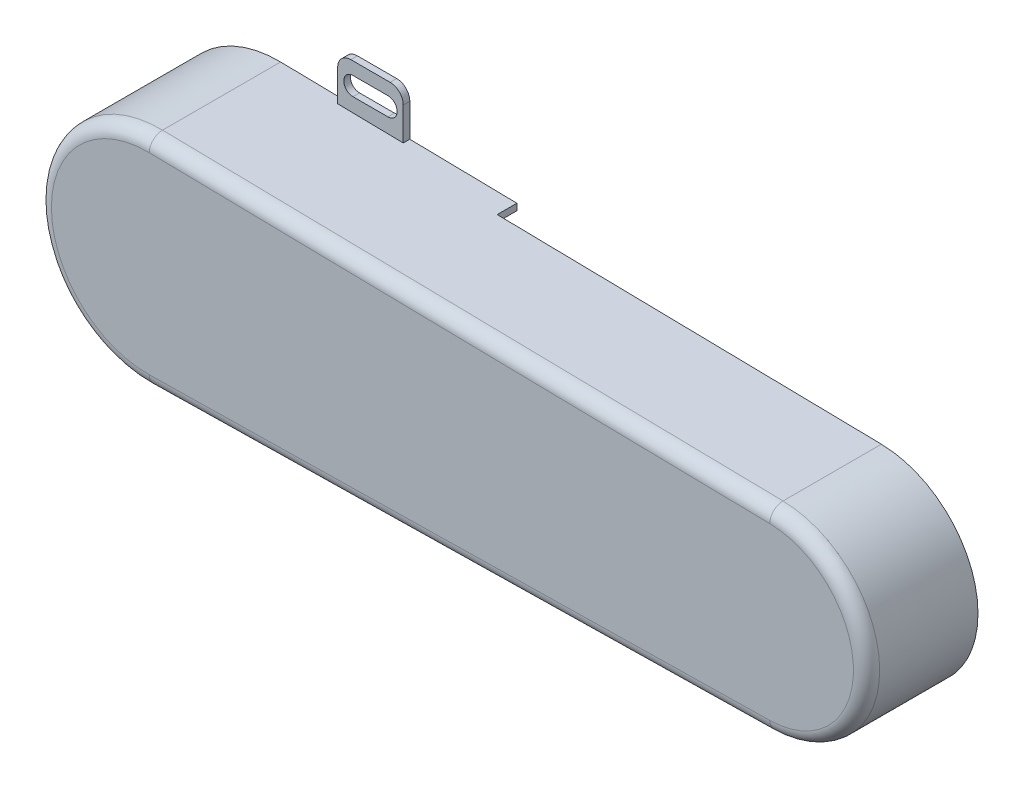
from build123d import *

# Parameters (mm, degrees)
EXTRUDE_1_DEPTH     = 30
SHELL_1_T           = -1.5
EXTRUDE_2_DEPTH     = 1.5
CUT_EXTRUDE_1_DEPTH = 1.5
FILLET_1_R          = 3
SKETCH_4_W          = 110
SKETCH_4_H          = 4.5
CUT_EXTRUDE_2_DEPTH = 30


with BuildPart() as part:
    # 草图1 → 凸台-拉伸1 (new body)
    with BuildSketch(Plane.XY):
        with BuildLine():
            Line((0.440140845, 24.99612522), (142.396126761, 22.496512698))
            ThreePointArc((142.396126761, 22.496512698), (164.5, 0), (142.396126761, -22.496512698))
            Line((142.396126761, -22.496512698), (0.440140845, -24.99612522))
            ThreePointArc((0.440140845, -24.99612522), (-25, 0), (0.440140845, 24.99612522))
        make_face()
    extrude(amount=EXTRUDE_1_DEPTH)

    # 抽壳1
    shell_1_openings = [part.faces().sort_by_distance(p)[0] for p in [
        (68.129004911, 0, 0),
    ]]
    offset(amount=SHELL_1_T, openings=shell_1_openings, kind=Kind.INTERSECTION)

    # 草图2 → 凸台-拉伸2 (add)
    with BuildSketch(Plane(origin=(0, 0, 0), x_dir=(-1, 0, 0), z_dir=(0, 0, -1))):
        Polygon((-30, 24.475624492), (-30, 35), (-15, 35), (-15, 24.739749936), align=None)
    extrude_2 = extrude(amount=-EXTRUDE_2_DEPTH)

    # 草图3 → 切除-拉伸1 (cut)
    with BuildSketch(Plane.XY.offset(1.5)):
        with BuildLine():
            Line((26.5, 27.9), (18.5, 27.9))
            ThreePointArc((18.5, 27.9), (16.4, 30), (18.5, 32.1))
            Line((18.5, 32.1), (26.5, 32.1))
            ThreePointArc((26.5, 32.1), (28.6, 30), (26.5, 27.9))
        make_face()
    cut_extrude_1 = extrude(amount=-CUT_EXTRUDE_1_DEPTH, mode=Mode.SUBTRACT)

    # 镜向1: 凸台-拉伸2, 切除-拉伸1 across plane
    add(extrude_2.mirror(Plane.ZX))
    add(cut_extrude_1.mirror(Plane.ZX), mode=Mode.SUBTRACT)

    # 圆角1
    fillet_1_edges = [part.edges().sort_by_distance(p)[0] for p in [
        (164.5, 0, 30),
        (71.418133803, 23.746318959, 30),
        (-23.5, 0, 28.5),
        (71.391725352, -22.246551446, 28.5),
        (163, 0, 28.5),
        (71.391725352, 22.246551446, 28.5),
        (30, 35, 0.75),
        (15, 35, 0.75),
        (-25, 0, 30),
        (15, -35, 0.75),
        (30, -35, 0.75),
        (71.418133803, -23.746318959, 30),
    ]]
    fillet(fillet_1_edges, radius=FILLET_1_R)

    # 草图4 → 切除-拉伸2 (cut, symmetric)
    with BuildSketch(Plane(origin=(0, 0, 0), x_dir=(1, 0, 0), z_dir=(0, 1, 0))):
        with Locations((109.5, -2.25)):
            Rectangle(SKETCH_4_W, SKETCH_4_H)
    extrude(amount=CUT_EXTRUDE_2_DEPTH, both=True, mode=Mode.SUBTRACT)


solid = part.part
